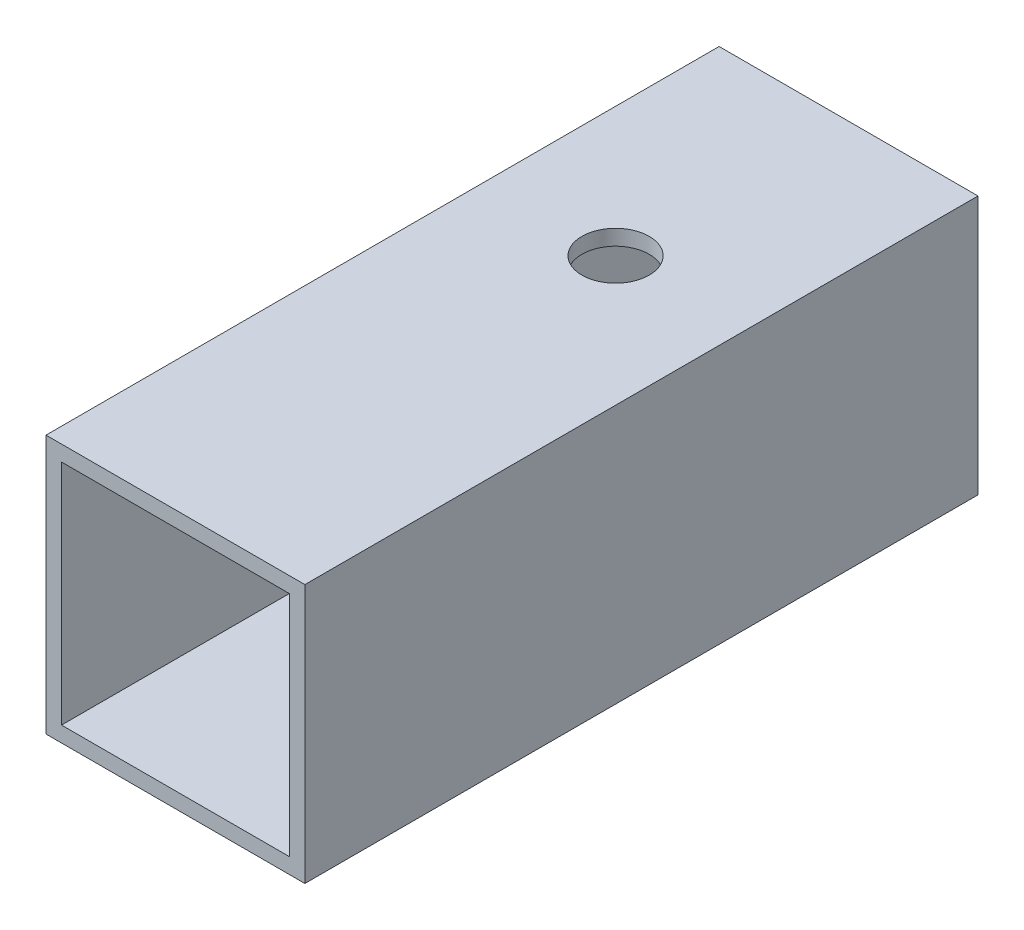
from build123d import *

# Parameters (mm, degrees)
SKETCH_1_W          = 50
SKETCH_1_H          = 50
SKETCH_1_W_2        = 44
SKETCH_1_H_2        = 44
EXTRUDE_1_DEPTH     = 130
SKETCH_5_R          = 6.5
CUT_EXTRUDE_1_DEPTH = 130


with BuildPart() as part:
    # 草图1 → 凸台-拉伸1 (new body)
    with BuildSketch(Plane.XY):
        with Locations((25, 25)):
            Rectangle(SKETCH_1_W, SKETCH_1_H)
        with Locations((25, 25)):
            Rectangle(SKETCH_1_W_2, SKETCH_1_H_2, mode=Mode.SUBTRACT)
    extrude(amount=EXTRUDE_1_DEPTH)

    # 草图5 → 切除-拉伸1 (cut)
    with BuildSketch(Plane(origin=(0, 50, 0), x_dir=(1, 0, 0), z_dir=(0, 1, 0))):
        with Locations(Location((25, -45, 0), (0, 0, 270))):
            Circle(SKETCH_5_R)
    extrude(amount=-CUT_EXTRUDE_1_DEPTH, mode=Mode.SUBTRACT)


solid = part.part
